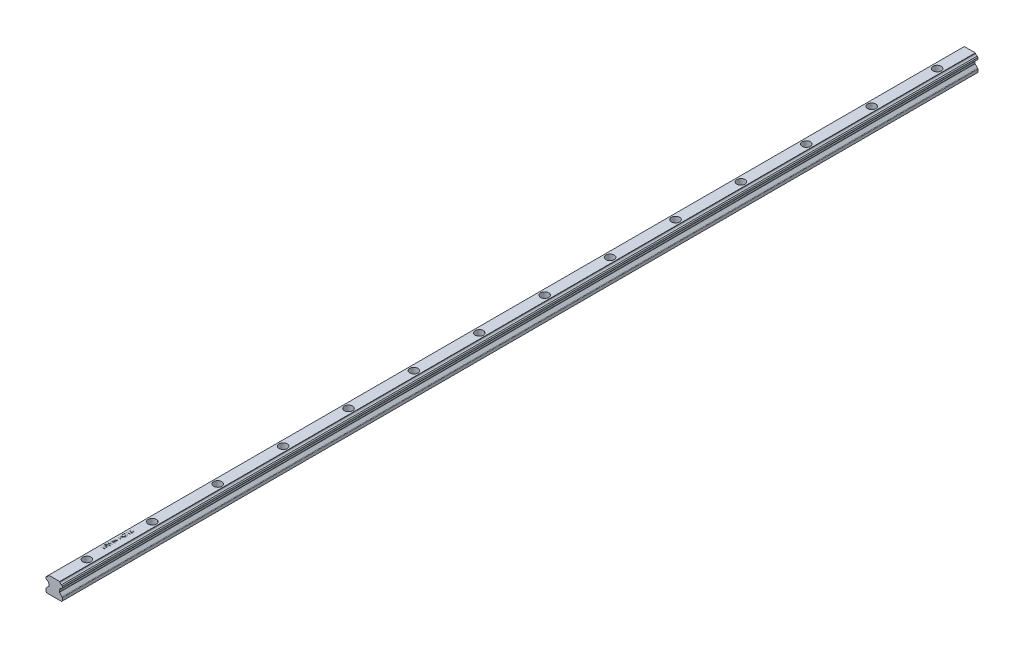
from build123d import *

# Parameters (mm, degrees)
BOSS_EXTRUDE1_DEPTH                                 = 840
CBORE_FOR_M4_HEX_SOCKET_HEAD_CAP_SCREW1_D           = 4.5
CBORE_FOR_M4_HEX_SOCKET_HEAD_CAP_SCREW1_CBORE_D     = 7.5
CBORE_FOR_M4_HEX_SOCKET_HEAD_CAP_SCREW1_CBORE_DEPTH = 5.3
LPATTERN1_COUNT                                     = 14
LPATTERN1_PITCH                                     = 60
SKETCH6_W                                           = 3.5
SKETCH6_H                                           = 0.314102564
CUT_EXTRUDE1_DEPTH                                  = 0.1


with BuildPart() as part:
    # Sketch1 → Boss-Extrude1 (new body)
    with BuildSketch(Plane.XY):
        with BuildLine():
            Line((7.5, 12.548994949), (6.730359225, 13.318635725))
            ThreePointArc((6.730359225, 13.318635725), (5.723905866, 13.746099326), (5.218323295, 14.715666114))
            ThreePointArc((5.218323295, 14.715666114), (5.180299299, 14.839173933), (5.104881891, 14.944113058))
            Line((5.104881891, 14.944113058), (5.04899495, 15))
            Line((5.04899495, 15), (-5.04899495, 15))
            Line((-5.04899495, 15), (-5.104881891, 14.944113058))
            ThreePointArc((-5.104881891, 14.944113058), (-5.180299299, 14.839173933), (-5.218323294, 14.715666114))
            ThreePointArc((-5.218323294, 14.715666114), (-5.723905866, 13.746099326), (-6.730359225, 13.318635725))
            Line((-6.730359225, 13.318635725), (-7.5, 12.548994949))
            Line((-7.5, 12.548994949), (-7.5, 11.011005051))
            Line((-7.5, 11.011005051), (-6.741857404, 10.252862454))
            ThreePointArc((-6.741857404, 10.252862454), (-5.724401564, 9.825237084), (-5.216972518, 8.845137289))
            ThreePointArc((-5.216972518, 8.845137289), (-5.179171399, 8.720266667), (-5.10319759, 8.614202641))
            Line((-5.10319759, 8.614202641), (-4.887157287, 8.398162338))
            ThreePointArc((-4.887157287, 8.398162338), (-4.800448187, 8.268392999), (-4.77, 8.115319626))
            Line((-4.77, 8.115319626), (-4.77, 6.553259018))
            ThreePointArc((-4.77, 6.553259018), (-4.800448187, 6.400185645), (-4.887157287, 6.270416306))
            Line((-4.887157287, 6.270416306), (-7.207106781, 3.950466812))
            ThreePointArc((-7.207106781, 3.950466812), (-7.423879533, 3.626043463), (-7.5, 3.243360031))
            Line((-7.5, 3.243360031), (-7.5, 0.7))
            Line((-7.5, 0.7), (-6.8, 0))
            Line((-6.8, 0), (6.8, 0))
            Line((6.8, 0), (7.5, 0.7))
            Line((7.5, 0.7), (7.5, 3.243360031))
            ThreePointArc((7.5, 3.243360031), (7.423879533, 3.626043463), (7.207106781, 3.950466812))
            Line((7.207106781, 3.950466812), (4.887157287, 6.270416306))
            ThreePointArc((4.887157287, 6.270416306), (4.800448187, 6.400185645), (4.77, 6.553259018))
            Line((4.77, 6.553259018), (4.77, 8.115319626))
            ThreePointArc((4.77, 8.115319626), (4.800448187, 8.268392999), (4.887157287, 8.398162338))
            Line((4.887157287, 8.398162338), (5.10319759, 8.614202641))
            ThreePointArc((5.10319759, 8.614202641), (5.179171399, 8.720266667), (5.216972518, 8.845137289))
            ThreePointArc((5.216972518, 8.845137289), (5.724401564, 9.825237084), (6.741857404, 10.252862454))
            Line((6.741857404, 10.252862454), (7.5, 11.011005051))
            Line((7.5, 11.011005051), (7.5, 12.548994949))
        make_face()
    extrude(amount=-BOSS_EXTRUDE1_DEPTH)

    # CBORE for M4 Hex Socket Head Cap Screw1 (through all)
    with Locations(Plane(origin=(0.291487344, 15, -3.466272926), x_dir=(-1, 0, 0), z_dir=(0, 1, 0))):
        with Locations((0.291487344, -26.533727074)):
            cbore_for_m4_hex_socket_head_cap_screw1 = CounterBoreHole(CBORE_FOR_M4_HEX_SOCKET_HEAD_CAP_SCREW1_D / 2, CBORE_FOR_M4_HEX_SOCKET_HEAD_CAP_SCREW1_CBORE_D / 2, CBORE_FOR_M4_HEX_SOCKET_HEAD_CAP_SCREW1_CBORE_DEPTH)

    # LPattern1: CBORE for M4 Hex Socket Head Cap Screw1 ×14
    with Locations(*[(0, 0, -i * LPATTERN1_PITCH) for i in range(1, LPATTERN1_COUNT)]):
        add(cbore_for_m4_hex_socket_head_cap_screw1, mode=Mode.SUBTRACT)

    # Sketch6 → Cut-Extrude1 (cut)
    with BuildSketch(Plane(origin=(0, 15, 0), x_dir=(1, 0, 0), z_dir=(0, 1, 0))):
        Polygon((-3.5, 46.403846154), (-3.5, 46.717948718), (-2.064102564, 46.717948718), (-2.064102564, 48.512820513), (-3.5, 48.512820513), (-3.5, 48.826923077), (0, 48.826923077), (0, 48.512820513), (-1.705128205, 48.512820513), (-1.705128205, 46.717948718), (0, 46.717948718), (0, 46.403846154), align=None)
        with Locations((-1.75, 49.881410256)):
            Rectangle(SKETCH6_W, SKETCH6_H)
        Polygon((-3.5, 50.576923077), (-3.5, 50.901542468), (-0.933193109, 51.586538462), (-3.5, 52.605268429), (-3.5, 52.650841346), (-0.950721154, 53.650641026), (-3.5, 54.339142628), (-3.5, 54.66025641), (0, 53.716546474), (0, 53.671674679), (-2.676883013, 52.618589744), (0, 51.552884615), (0, 51.508012821), align=None)
        with Locations((-1.75, 55.625)):
            Rectangle(SKETCH6_W, SKETCH6_H)
        Polygon((0, 56.544871795), (-3.5, 56.544871795), (-3.5, 56.610777244), (-0.745292468, 58.923076923), (-3.5, 58.923076923), (-3.5, 59.237179487), (0, 59.237179487), (0, 59.165665064), (-2.748397436, 56.858974359), (0, 56.858974359), align=None)
        Polygon((-3.5, 61.480769231), (-3.5, 61.794871795), (-2.064102564, 61.794871795), (-2.064102564, 63.58974359), (-3.5, 63.58974359), (-3.5, 63.903846154), (0, 63.903846154), (0, 63.58974359), (-1.705128205, 63.58974359), (-1.705128205, 61.794871795), (0, 61.794871795), (0, 61.480769231), align=None)
        with BuildLine():
            Line((-2.902644231, 68.076923077), (-2.647435897, 67.807692308))
            add(Edge.make_bspline(
                [(-2.647435897, 67.807692308), (-2.69328212, 67.758983227), (-2.783881335, 67.662726562), (-2.901244074, 67.50552662), (-3.002777003, 67.342170767), (-3.084772592, 67.172394867), (-3.149094254, 67.000650867), (-3.195850217, 66.829891913), (-3.225460377, 66.661223615), (-3.229016796, 66.549059313), (-3.230769231, 66.493790064)],
                knots=[0, 0, 0, 0, 1.089067066, 2.152164705, 3.18986567, 4.218445106, 5.218487318, 6.173592265, 7.100032889, 8, 8, 8, 8], degree=3))
            add(Edge.make_bspline(
                [(-3.230769231, 66.493790064), (-3.230355625, 66.459875364), (-3.229529486, 66.392133924), (-3.218985271, 66.29151198), (-3.203820407, 66.191945342), (-3.181878529, 66.093621968), (-3.15406947, 65.99635068), (-3.119284004, 65.900469793), (-3.078728771, 65.805800421), (-3.031866252, 65.713234402), (-2.980386575, 65.623493669), (-2.923337414, 65.538737672), (-2.862550889, 65.458421211), (-2.796491613, 65.384072004), (-2.725807311, 65.31519549), (-2.651770944, 65.250524789), (-2.572926872, 65.191265211), (-2.489599321, 65.138479571), (-2.403726867, 65.090811977), (-2.316037795, 65.049619777), (-2.227346143, 65.013809823), (-2.136984078, 64.986535862), (-2.045883197, 64.963434988), (-1.953566086, 64.947353752), (-1.859791669, 64.938257435), (-1.796993971, 64.936686944), (-1.765424679, 64.935897436)],
                knots=[0, 0, 0, 0, 1.028150113, 2.053633673, 3.06513288, 4.081487945, 5.106702018, 6.131327874, 7.172780699, 8.228344599, 9.276313556, 10.308389736, 11.324843658, 12.329040066, 13.321460474, 14.316307835, 15.308626991, 16.309440696, 17.305625405, 18.28535951, 19.246194545, 20.203493668, 21.145557131, 22.095268976, 23.042464743, 24, 24, 24, 24], degree=3))
            add(Edge.make_bspline(
                [(-1.765424679, 64.935897436), (-1.733154018, 64.936653631), (-1.668700816, 64.938163957), (-1.572504414, 64.947817154), (-1.477747832, 64.965772364), (-1.384282029, 64.989584114), (-1.291920993, 65.019856789), (-1.20076111, 65.057049303), (-1.110811241, 65.101355435), (-1.022964324, 65.152526704), (-0.937464192, 65.209036172), (-0.856251713, 65.271187356), (-0.780271995, 65.339084893), (-0.708415252, 65.411483836), (-0.641134974, 65.489043832), (-0.579242122, 65.572517364), (-0.521779643, 65.660735956), (-0.469378807, 65.753738745), (-0.42257144, 65.850542725), (-0.38094723, 65.949799156), (-0.346667976, 66.051827058), (-0.31872985, 66.156089724), (-0.295829559, 66.262463002), (-0.281097077, 66.371486803), (-0.270406246, 66.482359512), (-0.269624576, 66.557098144), (-0.269230769, 66.594751603)],
                knots=[0, 0, 0, 0, 0.935915162, 1.869274651, 2.799799983, 3.730201895, 4.664668062, 5.616159355, 6.583070886, 7.570012957, 8.562524459, 9.553461134, 10.53281078, 11.515274572, 12.509912756, 13.507571325, 14.526460018, 15.561318395, 16.601025881, 17.643204557, 18.680545676, 19.719612342, 20.772381578, 21.833430283, 22.908478249, 24, 24, 24, 24], degree=3))
            add(Edge.make_bspline(
                [(-0.269230769, 66.594751603), (-0.270178952, 66.640130135), (-0.272040863, 66.729238255), (-0.286546735, 66.860222075), (-0.309173205, 66.986034693), (-0.342412256, 67.106266531), (-0.384484705, 67.221353926), (-0.436513285, 67.330872414), (-0.497950569, 67.435124408), (-0.567552463, 67.533658668), (-0.645100929, 67.624132689), (-0.728035637, 67.706474768), (-0.817431068, 67.77785339), (-0.911954918, 67.840400707), (-1.012511326, 67.892097951), (-1.118540888, 67.934543829), (-1.230109213, 67.967076285), (-1.307200733, 67.980431374), (-1.346153846, 67.987179487)],
                knots=[0, 0, 0, 0, 1.130199668, 2.219330667, 3.279027493, 4.311506524, 5.322739849, 6.327972234, 7.327472899, 8.33386792, 9.329086447, 10.29244429, 11.240784345, 12.174119183, 13.111530729, 14.052100829, 15.015757696, 16, 16, 16, 16], degree=3))
            Line((-1.346153846, 67.987179487), (-1.346153846, 66.820512821))
            Line((-1.346153846, 66.820512821), (-1.705128205, 66.820512821))
            Line((-1.705128205, 66.820512821), (-1.705128205, 68.301282051))
            add(Edge.make_bspline(
                [(-1.705128205, 68.301282051), (-1.638220716, 68.299576203), (-1.507270675, 68.296237549), (-1.316300404, 68.272818634), (-1.13592871, 68.235002122), (-0.965965639, 68.18334181), (-0.806652046, 68.116466529), (-0.65782618, 68.035094001), (-0.520449499, 67.93792188), (-0.393400495, 67.828411438), (-0.280071283, 67.705511481), (-0.180465345, 67.572542861), (-0.09656273, 67.429285892), (-0.028302067, 67.275876085), (0.024971927, 67.112815651), (0.062743504, 66.939727272), (0.085373467, 66.756845671), (0.088264847, 66.631508994), (0.08974359, 66.567407853)],
                knots=[0, 0, 0, 0, 1.140356446, 2.231883559, 3.274166699, 4.278491846, 5.25512956, 6.21435461, 7.1637429, 8.11826594, 9.068280886, 10.0076534, 10.945064095, 11.891975133, 12.864533718, 13.863980011, 14.907571808, 16, 16, 16, 16], degree=3))
            add(Edge.make_bspline(
                [(0.08974359, 66.567407853), (0.089174469, 66.527897717), (0.088051978, 66.449970996), (0.080074631, 66.334880068), (0.067794054, 66.222962448), (0.049248931, 66.114234439), (0.026534277, 66.008296097), (-0.002552442, 65.905676512), (-0.036221141, 65.80598477), (-0.074516815, 65.709066784), (-0.118888472, 65.615802237), (-0.168198111, 65.52577572), (-0.222191472, 65.438489595), (-0.281802318, 65.35453843), (-0.346584778, 65.273484808), (-0.416668697, 65.195851364), (-0.491839816, 65.121203486), (-0.545218826, 65.074443023), (-0.572115385, 65.05088141)],
                knots=[0, 0, 0, 0, 1.107784379, 2.184907829, 3.233506516, 4.263428166, 5.276301166, 6.270063455, 7.25232949, 8.225834625, 9.190232166, 10.146266622, 11.1027726, 12.066435141, 13.031522626, 14.010570082, 14.99756817, 16, 16, 16, 16], degree=3))
            add(Edge.make_bspline(
                [(-0.572115385, 65.05088141), (-0.614786038, 65.016695478), (-0.699419055, 64.948891066), (-0.835018999, 64.861612909), (-0.975420859, 64.787211506), (-1.121015488, 64.726843684), (-1.271666701, 64.679705598), (-1.427181992, 64.645899345), (-1.587761622, 64.626092056), (-1.696426887, 64.623238518), (-1.751402244, 64.621794872)],
                knots=[0, 0, 0, 0, 1.023165419, 2.029347347, 3.013907458, 3.994755782, 4.975994455, 5.96558838, 6.970761222, 8, 8, 8, 8], degree=3))
            add(Edge.make_bspline(
                [(-1.751402244, 64.621794872), (-1.792568496, 64.62232711), (-1.874377804, 64.623384821), (-1.99583511, 64.636210339), (-2.115135808, 64.654611751), (-2.232182344, 64.681658827), (-2.347053012, 64.715755013), (-2.45980069, 64.758308794), (-2.570493643, 64.807852572), (-2.67836343, 64.865442289), (-2.782003044, 64.929511026), (-2.880905313, 64.999118682), (-2.973467332, 65.074802367), (-3.059903521, 65.156782462), (-3.141494975, 65.243406392), (-3.216537375, 65.336492693), (-3.286205011, 65.434631029), (-3.349159221, 65.538582169), (-3.405727075, 65.6467058), (-3.455315154, 65.758766886), (-3.496298775, 65.874724704), (-3.531072472, 65.993712261), (-3.556787635, 66.11662974), (-3.575436374, 66.242585283), (-3.588196976, 66.372235393), (-3.589223231, 66.459871423), (-3.58974359, 66.504306891)],
                knots=[0, 0, 0, 0, 1.00895651, 2.005089799, 2.991467152, 3.967318338, 4.948153826, 5.927364234, 6.919980553, 7.91976625, 8.923240147, 9.905815003, 10.88314567, 11.851989312, 12.825009789, 13.798721852, 14.781296708, 15.773896486, 16.776076962, 17.771600213, 18.775744723, 19.78957137, 20.808953803, 21.851964491, 22.910847925, 24, 24, 24, 24], degree=3))
            add(Edge.make_bspline(
                [(-3.58974359, 66.504306891), (-3.589164098, 66.540545135), (-3.588015034, 66.612401313), (-3.580050386, 66.719327046), (-3.567426505, 66.82460006), (-3.550199718, 66.92837645), (-3.526736028, 67.030302816), (-3.498657743, 67.130669522), (-3.46596592, 67.229622058), (-3.426977074, 67.326850307), (-3.382723449, 67.423008023), (-3.332910027, 67.518629864), (-3.276685022, 67.61338911), (-3.213881487, 67.707450091), (-3.145578069, 67.801405949), (-3.069821245, 67.893770591), (-2.989598489, 67.986773536), (-2.931916305, 68.04657535), (-2.902644231, 68.076923077)],
                knots=[0, 0, 0, 0, 0.985871117, 1.954866573, 2.915460327, 3.869826059, 4.81536089, 5.759505086, 6.70452669, 7.649098992, 8.607881297, 9.583363685, 10.581137262, 11.603961102, 12.659522466, 13.73993555, 14.853081303, 16, 16, 16, 16], degree=3))
        make_face()
        Polygon((-3.5, 69.449018429), (-3.5, 70.096153846), (0, 70.096153846), (0, 69.782051282), (-3.141025641, 69.782051282), (-3.141025641, 69.243589744), align=None)
        with BuildLine():
            Line((-3.5, 73.596153846), (-3.141025641, 73.596153846))
            Line((-3.141025641, 73.596153846), (-3.141025641, 72.405649038))
            Line((-3.141025641, 72.405649038), (-2.220452724, 72.217047276))
            add(Edge.make_bspline(
                [(-2.220452724, 72.217047276), (-2.230682996, 72.25410315), (-2.25050253, 72.325893046), (-2.2725083, 72.431852907), (-2.285773744, 72.53244511), (-2.287585055, 72.597720481), (-2.288461538, 72.629306891)],
                knots=[0, 0, 0, 0, 1.100273476, 2.13160584, 3.095893838, 4, 4, 4, 4], degree=3))
            add(Edge.make_bspline(
                [(-2.288461538, 72.629306891), (-2.28764354, 72.668397805), (-2.28603515, 72.745260309), (-2.269673986, 72.857544614), (-2.245976174, 72.96527195), (-2.209465207, 73.066851732), (-2.164878805, 73.163891055), (-2.108721258, 73.254723386), (-2.04315746, 73.34062356), (-1.968525078, 73.420997879), (-1.885534459, 73.493570878), (-1.795933934, 73.556634421), (-1.701678739, 73.611677196), (-1.600559725, 73.654605621), (-1.494484031, 73.689639403), (-1.382227183, 73.712740767), (-1.264785773, 73.728171477), (-1.18448027, 73.729891917), (-1.143529647, 73.730769231)],
                knots=[0, 0, 0, 0, 1.052805225, 2.070078116, 3.052532748, 4.020689046, 4.973125432, 5.925915817, 6.89216474, 7.881560752, 8.877013184, 9.857446635, 10.830895175, 11.812622661, 12.812548702, 13.836681939, 14.896847428, 16, 16, 16, 16], degree=3))
            add(Edge.make_bspline(
                [(-1.143529647, 73.730769231), (-1.115007605, 73.730103556), (-1.058348972, 73.728781204), (-0.974202158, 73.7220714), (-0.891849045, 73.709103007), (-0.811440613, 73.69190289), (-0.732901554, 73.668941583), (-0.65579213, 73.642084161), (-0.580956685, 73.608702163), (-0.508064701, 73.571694489), (-0.437950402, 73.530715464), (-0.372294905, 73.484635462), (-0.309599937, 73.436755685), (-0.251727444, 73.384438189), (-0.198452948, 73.328277796), (-0.149513072, 73.268586987), (-0.104029493, 73.205907167), (-0.063861909, 73.139251137), (-0.026898788, 73.070108867), (0.003424705, 72.997480593), (0.030535245, 72.923019908), (0.05214477, 72.845655028), (0.069077325, 72.765561217), (0.080577925, 72.682606441), (0.088954363, 72.597225771), (0.08947872, 72.539350758), (0.08974359, 72.510116186)],
                knots=[0, 0, 0, 0, 1.056393913, 2.098511576, 3.122979385, 4.141471433, 5.141222888, 6.151259816, 7.162667642, 8.172852865, 9.177685681, 10.166741883, 11.141342384, 12.097242845, 13.052202613, 14.005160326, 14.953864445, 15.917140761, 16.884916217, 17.854238259, 18.828761908, 19.81781811, 20.826036654, 21.857789401, 22.917898972, 24, 24, 24, 24], degree=3))
            add(Edge.make_bspline(
                [(0.08974359, 72.510116186), (0.089050894, 72.475242894), (0.087688097, 72.406633813), (0.073496095, 72.30610057), (0.053035464, 72.209432256), (0.022721931, 72.117043177), (-0.016971483, 72.029318648), (-0.064133263, 71.945002475), (-0.12027864, 71.865139718), (-0.184894072, 71.790276377), (-0.255892818, 71.721460371), (-0.332202561, 71.65905751), (-0.413920487, 71.604193873), (-0.500780871, 71.556670445), (-0.592629648, 71.516184815), (-0.689749822, 71.484366409), (-0.791650601, 71.45868899), (-0.861804004, 71.447825441), (-0.897435897, 71.442307692)],
                knots=[0, 0, 0, 0, 1.046872515, 2.059598001, 3.044168548, 4.012104806, 4.973680974, 5.932408326, 6.910122221, 7.900780896, 8.89867654, 9.876692837, 10.858029398, 11.85084981, 12.847361615, 13.868568023, 14.917415949, 16, 16, 16, 16], degree=3))
            Line((-0.897435897, 71.442307692), (-0.897435897, 71.756410256))
            add(Edge.make_bspline(
                [(-0.897435897, 71.756410256), (-0.86405597, 71.764133979), (-0.799897896, 71.778979402), (-0.709812799, 71.811649494), (-0.62950762, 71.851206459), (-0.558491359, 71.899340396), (-0.495464081, 71.955133792), (-0.43989307, 72.019990731), (-0.389697273, 72.092289811), (-0.347784769, 72.17267219), (-0.312479137, 72.257640252), (-0.287283878, 72.346063351), (-0.272032646, 72.436668904), (-0.270168243, 72.497671524), (-0.269230769, 72.528345353)],
                knots=[0, 0, 0, 0, 1.13623081, 2.183898708, 3.172478118, 4.09966615, 5.022692284, 5.957376522, 6.927682873, 7.937366477, 8.960015386, 9.976409503, 10.982481913, 12, 12, 12, 12], degree=3))
            add(Edge.make_bspline(
                [(-0.269230769, 72.528345353), (-0.270058415, 72.558301256), (-0.271688055, 72.617284674), (-0.284028564, 72.704132513), (-0.303533592, 72.787735767), (-0.33085902, 72.868242843), (-0.367008958, 72.945258145), (-0.411417074, 73.018672781), (-0.462975425, 73.089532607), (-0.521904738, 73.1559727), (-0.586881759, 73.216808942), (-0.656357238, 73.270565902), (-0.730474586, 73.315342595), (-0.807947606, 73.353076763), (-0.889626199, 73.381730046), (-0.975127364, 73.402171031), (-1.064662347, 73.414174089), (-1.125731657, 73.415825269), (-1.156850962, 73.416666667)],
                knots=[0, 0, 0, 0, 1.027268864, 2.022700798, 3.002744649, 3.968653148, 4.933396556, 5.915045722, 6.907600446, 7.935526002, 8.956456544, 9.95700807, 10.942805781, 11.92166854, 12.907987664, 13.905483474, 14.932689774, 16, 16, 16, 16], degree=3))
            add(Edge.make_bspline(
                [(-1.156850962, 73.416666667), (-1.184930032, 73.416028195), (-1.239659043, 73.414783746), (-1.320009695, 73.404010642), (-1.396158478, 73.386014341), (-1.468436727, 73.360391264), (-1.536613353, 73.328412845), (-1.600538112, 73.288262971), (-1.660812066, 73.241651258), (-1.715884112, 73.187233139), (-1.766793088, 73.12803749), (-1.810034281, 73.062543866), (-1.846807397, 72.992500701), (-1.876936465, 72.917778197), (-1.900936575, 72.838284311), (-1.917523378, 72.753976228), (-1.92744867, 72.664834733), (-1.928795087, 72.603859089), (-1.929487179, 72.572516026)],
                knots=[0, 0, 0, 0, 1.045723156, 2.038222538, 3.013889863, 3.95567481, 4.890389958, 5.81331128, 6.76251276, 7.723027653, 8.692928204, 9.666105983, 10.639751036, 11.635719707, 12.66315958, 13.728667616, 14.832476222, 16, 16, 16, 16], degree=3))
            add(Edge.make_bspline(
                [(-1.929487179, 72.572516026), (-1.928906588, 72.545387097), (-1.927707815, 72.489372742), (-1.918881318, 72.403449915), (-1.904642024, 72.313158192), (-1.885055776, 72.218843696), (-1.859424699, 72.120223188), (-1.828710199, 72.017504787), (-1.7919882, 71.910472521), (-1.764255986, 71.838354796), (-1.75, 71.801282051)],
                knots=[0, 0, 0, 0, 0.817624296, 1.688186739, 2.600797293, 3.572016777, 4.590301741, 5.671205678, 6.80286297, 8, 8, 8, 8], degree=3))
            Line((-1.75, 71.801282051), (-3.5, 72.16025641))
            Line((-3.5, 72.16025641), (-3.5, 73.596153846))
        make_face()
    extrude(amount=-CUT_EXTRUDE1_DEPTH, mode=Mode.SUBTRACT)


solid = part.part
